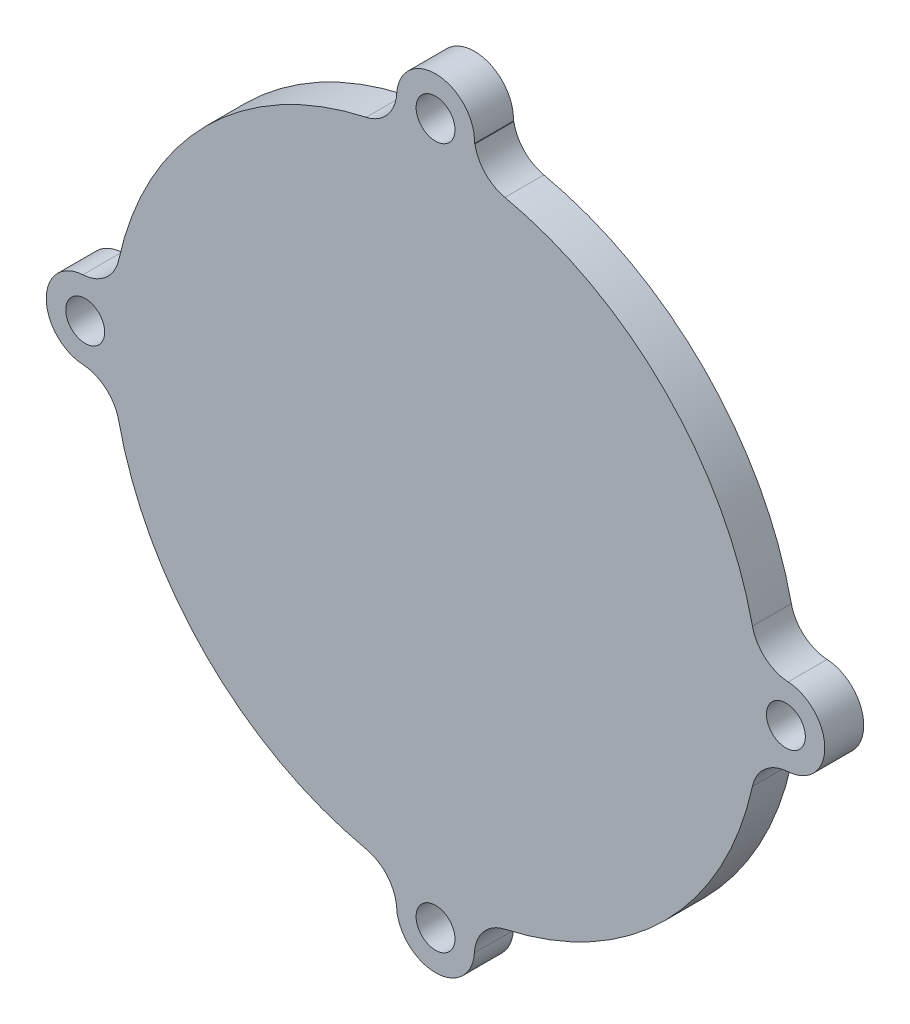
SolidWorks part; units mm, degrees
material "铜"
ref_plane "前视基准面" through (0, 0, 0) normal (0, 0, 1) x (1, 0, 0)
ref_plane "上视基准面" through (0, 0, 0) normal (0, 1, 0) x (1, 0, 0)
ref_plane "右视基准面" through (0, 0, 0) normal (1, 0, 0) x (0, 0, -1)
sketch "草图1" plane through (0, 0, 0) normal (0, 0, 1) x (1, 0, 0)
  line L0 (-27, 0) -> (27, 0) construction
  line L1 (0, 27) -> (0, -27) construction
  arc A1 (-5.3479, 24.4213) -> (-24.4213, 5.3479) centre (0, 0) ccw
  circle A2 centre (0, 27) radius 1.5
  arc A6 (2.9954, 26.8333) -> (-2.9954, 26.8333) centre (0, 27) ccw
  arc A7 (-5.3479, 24.4213) -> (-2.9948, 27.1759) centre (-5.9897, 27.3519) ccw
  arc A8 (5.3479, 24.4213) -> (2.9948, 27.1759) centre (5.9897, 27.3519) cw
  arc A9 (-2.9954, 26.8333) -> (-3.0356, 26.8288) centre (0, 0) ccw
  arc A10 (3.0356, 26.8288) -> (2.9954, 26.8333) centre (0, 0) ccw
  circle A11 centre (27, 0) radius 1.5
  arc A12 (26.8333, -2.9954) -> (26.8333, 2.9954) centre (27, 0) ccw
  arc A13 (24.4213, -5.3479) -> (27.1759, -2.9948) centre (27.3519, -5.9897) cw
  arc A14 (24.4213, 5.3479) -> (27.1759, 2.9948) centre (27.3519, 5.9897) ccw
  circle A15 centre (0, -27) radius 1.5
  arc A16 (-2.9954, -26.8333) -> (2.9954, -26.8333) centre (0, -27) ccw
  arc A17 (-5.3479, -24.4213) -> (-2.9948, -27.1759) centre (-5.9897, -27.3519) cw
  arc A18 (5.3479, -24.4213) -> (2.9948, -27.1759) centre (5.9897, -27.3519) ccw
  circle A19 centre (-27, 0) radius 1.5
  arc A20 (-26.8333, 2.9954) -> (-26.8333, -2.9954) centre (-27, 0) ccw
  arc A21 (-24.4213, 5.3479) -> (-27.1759, 2.9948) centre (-27.3519, 5.9897) cw
  arc A22 (-24.4213, -5.3479) -> (-27.1759, -2.9948) centre (-27.3519, -5.9897) ccw
  arc A23 (-24.4213, -5.3479) -> (-5.3479, -24.4213) centre (0, 0) ccw
  arc A24 (24.4213, 5.3479) -> (5.3479, 24.4213) centre (0, 0) ccw
  arc A25 (5.3479, -24.4213) -> (24.4213, -5.3479) centre (0, 0) ccw
  circle A26 centre (0, 0) radius 27 construction
  point P50 (0, 0)
  dimension "D1" = 4
  dimension "D2" = 3
  dimension "D3" = 54
  dimension "D6" = 50
  dimension "D7" = 6
  dimension "D8" = 3
extrude "凸台-拉伸1" add sketch "草图1" along normal blind 3
